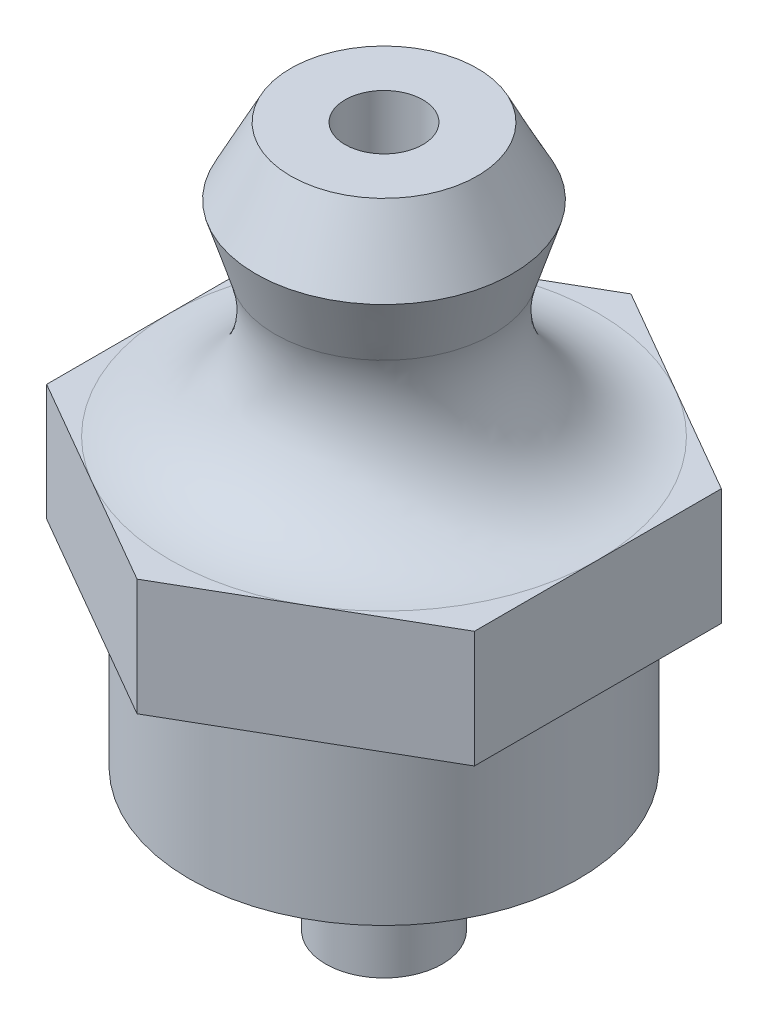
from build123d import *

# Parameters (mm, degrees)
EXTRUDE_1_DEPTH = 3


with BuildPart() as part:
    # 草图1 → 旋转2 (revolve)
    with BuildSketch(Plane.XY, mode=Mode.PRIVATE) as revolve_2_sk:
        with BuildLine():
            Line((-1, 18), (-2.4, 18))
            Line((-2.4, 18), (-3.3, 16.271116086))
            Line((-3.3, 16.271116086), (-2.8, 14.675583457))
            ThreePointArc((-2.8, 14.675583457), (-3.219653878, 12.154380629), (-5.5, 11))
            Line((-5.5, 11), (-5.5, 8))
            Line((-5.5, 8), (-5, 8))
            Line((-5, 8), (-5, 3.643969354))
            Line((-5, 3.643969354), (-1.5, 1.821984677))
            Line((-1.5, 1.821984677), (-1.5, 0))
            Line((-1.5, 0), (-1, 0))
            Line((-1, 0), (-1, 18))
        make_face()
    revolve(revolve_2_sk.sketch.rotate(Axis((0, 0, 0), (0, -1, 0)), 270), axis=Axis((0, 0, 0), (0, -1, 0)))

    # 草图2 → 拉伸1 (add)
    with BuildSketch(Plane.XZ.offset(-8)):
        Polygon((-5.5, 3.175426481), (-5.5, -3.175426481), (0, -6.350852961), (5.5, -3.175426481), (5.5, 3.175426481), (0, 6.350852961), align=None)
    extrude(amount=-EXTRUDE_1_DEPTH)


solid = part.part
